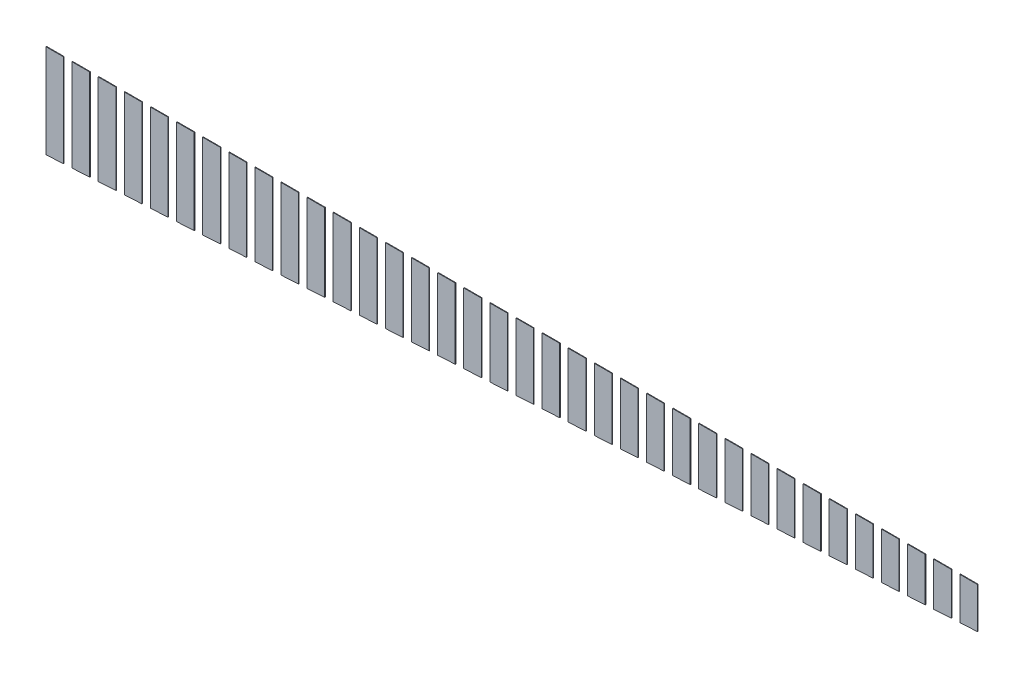
from build123d import *

# Parameters (mm, degrees)
SKETCH1_W           = 178.5
SKETCH1_H           = 19
BOSS_EXTRUDE1_DEPTH = 0.1
SKETCH2_W           = 214.462169904
SKETCH2_H           = 58.553279971
CUT_EXTRUDE1_DEPTH  = 10


with BuildPart() as part:
    # Sketch1 → Boss-Extrude1 (new body)
    with BuildSketch(Plane.XY):
        Rectangle(SKETCH1_W, SKETCH1_H)
    extrude(amount=BOSS_EXTRUDE1_DEPTH)

    # Sketch2 → Cut-Extrude1 (cut)
    with BuildSketch(Plane.XY.offset(0.1)):
        with Locations((2.468770954, -3.863989357)):
            Rectangle(SKETCH2_W, SKETCH2_H)
        Polygon((-77.71, 7.7), (-74.81, 7.7), (-74.81, -7.547475845), (-77.71, -7.711642006), align=None, mode=Mode.SUBTRACT)
        Polygon((-73.41, 7.7), (-70.51, 7.7), (-70.51, -7.304057054), (-73.41, -7.468223215), align=None, mode=Mode.SUBTRACT)
        Polygon((-69.11, 7.7), (-66.21, 7.7), (-66.21, -7.060638263), (-69.11, -7.224804424), align=None, mode=Mode.SUBTRACT)
        Polygon((-64.81, 7.7), (-61.91, 7.7), (-61.91, -6.817219472), (-64.81, -6.981385633), align=None, mode=Mode.SUBTRACT)
        Polygon((-60.51, 7.7), (-57.61, 7.7), (-57.61, -6.573800681), (-60.51, -6.737966842), align=None, mode=Mode.SUBTRACT)
        Polygon((-56.21, 7.7), (-53.31, 7.7), (-53.31, -6.33038189), (-56.21, -6.494548051), align=None, mode=Mode.SUBTRACT)
        Polygon((-51.91, 7.7), (-49.01, 7.7), (-49.01, -6.086963099), (-51.91, -6.25112926), align=None, mode=Mode.SUBTRACT)
        Polygon((-47.61, 7.7), (-44.71, 7.7), (-44.71, -5.843544308), (-47.61, -6.007710469), align=None, mode=Mode.SUBTRACT)
        Polygon((-43.31, 7.7), (-40.41, 7.7), (-40.41, -5.600125517), (-43.31, -5.764291678), align=None, mode=Mode.SUBTRACT)
        Polygon((-39.01, 7.7), (-36.11, 7.7), (-36.11, -5.356706726), (-39.01, -5.520872887), align=None, mode=Mode.SUBTRACT)
        Polygon((-34.71, 7.7), (-31.81, 7.7), (-31.81, -5.113287935), (-34.71, -5.277454096), align=None, mode=Mode.SUBTRACT)
        Polygon((-30.41, 7.7), (-27.51, 7.7), (-27.51, -4.869869144), (-30.41, -5.034035305), align=None, mode=Mode.SUBTRACT)
        Polygon((-26.11, 7.7), (-23.21, 7.7), (-23.21, -4.626450353), (-26.11, -4.790616514), align=None, mode=Mode.SUBTRACT)
        Polygon((-21.81, 7.7), (-18.91, 7.7), (-18.91, -4.383031561), (-21.81, -4.547197723), align=None, mode=Mode.SUBTRACT)
        Polygon((-17.51, 7.7), (-14.61, 7.7), (-14.61, -4.13961277), (-17.51, -4.303778932), align=None, mode=Mode.SUBTRACT)
        Polygon((-13.21, 7.7), (-10.31, 7.7), (-10.31, -3.896193979), (-13.21, -4.060360141), align=None, mode=Mode.SUBTRACT)
        Polygon((-8.91, 7.7), (-6.01, 7.7), (-6.01, -3.652775188), (-8.91, -3.81694135), align=None, mode=Mode.SUBTRACT)
        Polygon((-4.61, 7.7), (-1.71, 7.7), (-1.71, -3.409356397), (-4.61, -3.573522559), align=None, mode=Mode.SUBTRACT)
        Polygon((-0.31, 7.7), (2.59, 7.7), (2.59, -3.165937606), (-0.31, -3.330103768), align=None, mode=Mode.SUBTRACT)
        Polygon((3.99, 7.7), (6.89, 7.7), (6.89, -2.922518815), (3.99, -3.086684977), align=None, mode=Mode.SUBTRACT)
        Polygon((8.29, 7.7), (11.19, 7.7), (11.19, -2.679100024), (8.29, -2.843266186), align=None, mode=Mode.SUBTRACT)
        Polygon((12.59, 7.7), (15.49, 7.7), (15.49, -2.435681233), (12.59, -2.599847395), align=None, mode=Mode.SUBTRACT)
        Polygon((16.89, 7.7), (19.79, 7.7), (19.79, -2.192262442), (16.89, -2.356428604), align=None, mode=Mode.SUBTRACT)
        Polygon((21.19, 7.7), (24.09, 7.7), (24.09, -1.948843651), (21.19, -2.113009813), align=None, mode=Mode.SUBTRACT)
        Polygon((25.49, 7.7), (28.39, 7.7), (28.39, -1.70542486), (25.49, -1.869591022), align=None, mode=Mode.SUBTRACT)
        Polygon((29.79, 7.7), (32.69, 7.7), (32.69, -1.462006069), (29.79, -1.626172231), align=None, mode=Mode.SUBTRACT)
        Polygon((34.09, 7.7), (36.99, 7.7), (36.99, -1.218587278), (34.09, -1.38275344), align=None, mode=Mode.SUBTRACT)
        Polygon((38.39, 7.7), (41.29, 7.7), (41.29, -0.975168487), (38.39, -1.139334649), align=None, mode=Mode.SUBTRACT)
        Polygon((42.69, 7.7), (45.59, 7.7), (45.59, -0.731749696), (42.69, -0.895915858), align=None, mode=Mode.SUBTRACT)
        Polygon((46.99, 7.7), (49.89, 7.7), (49.89, -0.488330905), (46.99, -0.652497067), align=None, mode=Mode.SUBTRACT)
        Polygon((51.29, 7.7), (54.19, 7.7), (54.19, -0.244912114), (51.29, -0.409078276), align=None, mode=Mode.SUBTRACT)
        Polygon((55.59, 7.7), (58.49, 7.7), (58.49, -0.001493323), (55.59, -0.165659485), align=None, mode=Mode.SUBTRACT)
        Polygon((59.89, 7.7), (62.79, 7.7), (62.79, 0.241925468), (59.89, 0.077759306), align=None, mode=Mode.SUBTRACT)
        Polygon((64.19, 7.7), (67.09, 7.7), (67.09, 0.485344259), (64.19, 0.321178097), align=None, mode=Mode.SUBTRACT)
        Polygon((68.49, 7.7), (71.39, 7.7), (71.39, 0.72876305), (68.49, 0.564596888), align=None, mode=Mode.SUBTRACT)
        Polygon((72.79, 7.7), (75.69, 7.7), (75.69, 0.972181841), (72.79, 0.808015679), align=None, mode=Mode.SUBTRACT)
    extrude(amount=-CUT_EXTRUDE1_DEPTH, mode=Mode.SUBTRACT)


solid = part.part
